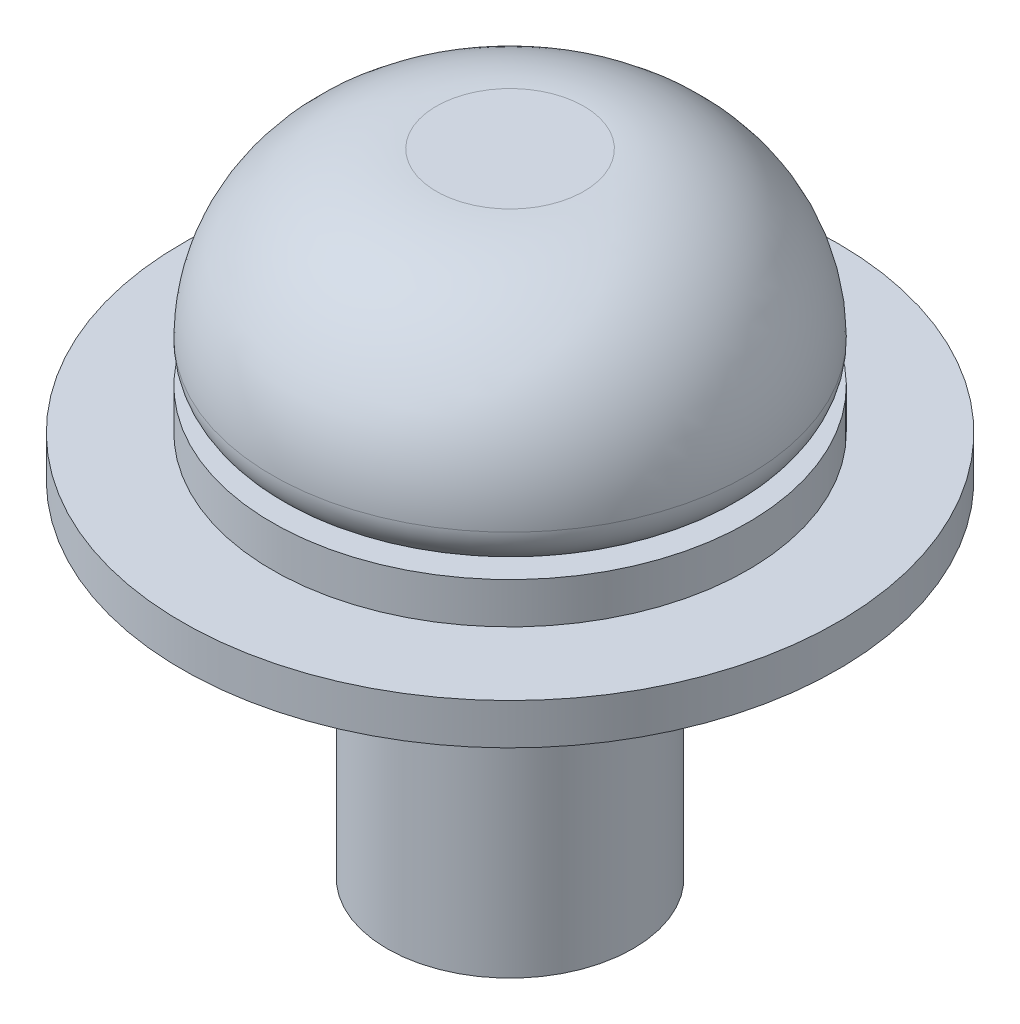
from build123d import *


with BuildPart() as part:
    # Sketch1 → Revolve1 (revolve)
    with BuildSketch(Plane(origin=(0, 0, 0), x_dir=(0, 0, -1), z_dir=(1, 0, 0)), mode=Mode.PRIVATE) as revolve1_sk:
        with BuildLine():
            Line((0, -4.2), (-1.5, -4.2))
            Line((-1.5, -4.2), (-1.5, 0))
            Line((-1.5, 0), (-4, 0))
            Line((-4, 0), (-4, 0.5))
            Line((-4, 0.5), (-2.9, 0.5))
            Line((-2.9, 0.5), (-2.9, 1))
            Line((-2.9, 1), (-2.4, 1))
            ThreePointArc((-2.4, 1), (-2.753553391, 1.146446609), (-2.9, 1.5))
            ThreePointArc((-2.9, 1.5), (-2.314213562, 2.914213562), (-0.9, 3.5))
            Line((-0.9, 3.5), (0, 3.5))
            Line((0, 3.5), (0, -4.2))
        make_face()
    revolve(revolve1_sk.sketch.rotate(Axis((0, 3.5, 0), (0, -1, 0)), 180), axis=Axis((0, 3.5, 0), (0, -1, 0)))


solid = part.part
